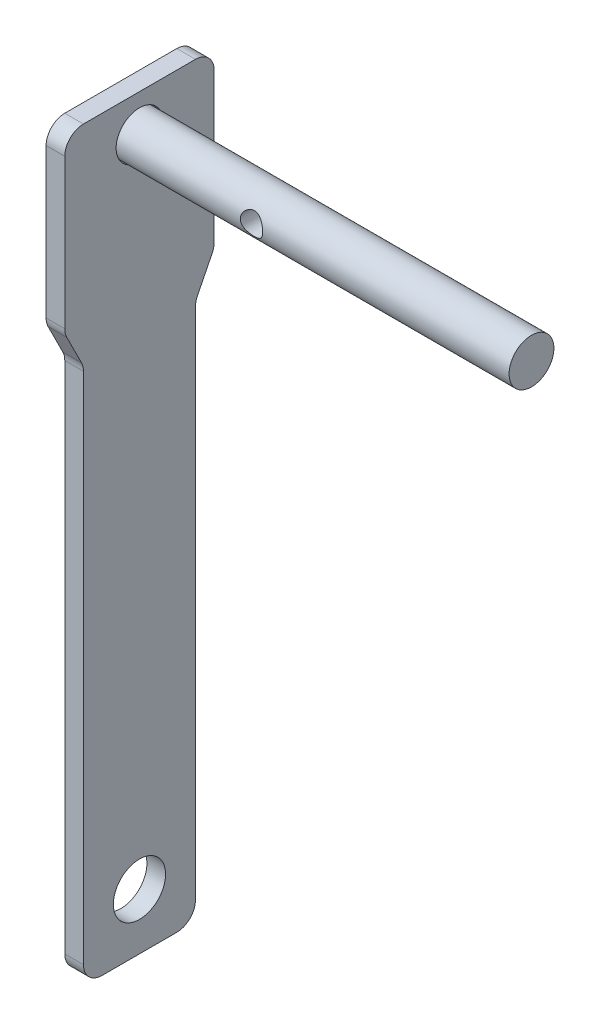
from build123d import *

# Parameters (mm, degrees)
SWEEP_1_PROFILE_R   = 6
SKETCH_4_R          = 3
CUT_EXTRUDE_2_DEPTH = 40
SKETCH_6_R          = 7
SKETCH_6_R_2        = 6.25
EXTRUDE_2_DEPTH     = 5
FILLET_1_R          = 5


with BuildPart() as part:
    # 扫描1: sweep along a path in 草图1
    with BuildLine(Plane.XY) as sweep_1_path:
        Line((110, -190), (220, -190))
    # 扫描1 profile (on start of the path) → 扫描1 (sweep)
    with BuildSketch(Plane(origin=(110, -190, 0), x_dir=(0, 0, 1), z_dir=(1, 0, 0))):
        Circle(SWEEP_1_PROFILE_R)
    sweep(path=sweep_1_path.line)

    # 草图4 → 切除-拉伸2 (cut, symmetric)
    with BuildSketch(Plane.XY):
        with Locations((151, -190)):
            Circle(SKETCH_4_R)
    extrude(amount=CUT_EXTRUDE_2_DEPTH, both=True, mode=Mode.SUBTRACT)


with BuildPart() as body_2:
    # 草图6 → 凸台-拉伸2 (new body)
    with BuildSketch(Plane.ZY.offset(-110)):
        with BuildLine():
            Line((-19.472135955, -227.236067977), (-15.527864045, -235.124611797))
            ThreePointArc((-15.527864045, -235.124611797), (-15.133755053, -236.211915172), (-15, -237.360679775))
            Line((-15, -237.360679775), (-15, -380))
            Line((-15, -380), (15, -380))
            Line((15, -380), (15, -237.360679775))
            ThreePointArc((15, -237.360679775), (15.133755053, -236.211915172), (15.527864045, -235.124611797))
            Line((15.527864045, -235.124611797), (19.472135955, -227.236067977))
            ThreePointArc((19.472135955, -227.236067977), (19.866244947, -226.148764603), (20, -225))
            Line((20, -225), (20, -185))
            ThreePointArc((20, -185), (18.535533906, -181.464466094), (15, -180))
            Line((15, -180), (-15, -180))
            ThreePointArc((-15, -180), (-18.535533906, -181.464466094), (-20, -185))
            Line((-20, -185), (-20, -225))
            ThreePointArc((-20, -225), (-19.866244947, -226.148764603), (-19.472135955, -227.236067977))
        make_face()
        with Locations((0, -365)):
            Circle(SKETCH_6_R, mode=Mode.SUBTRACT)
        with Locations((0, -190)):
            Circle(SKETCH_6_R_2, mode=Mode.SUBTRACT)
    extrude(amount=-EXTRUDE_2_DEPTH)

    # 圆角1
    fillet_1_edges = [body_2.edges().sort_by_distance(p)[0] for p in [
        (112.5, -380, 15),
        (112.5, -380, -15),
    ]]
    fillet(fillet_1_edges, radius=FILLET_1_R)


solid = Compound([part.part, body_2.part])
